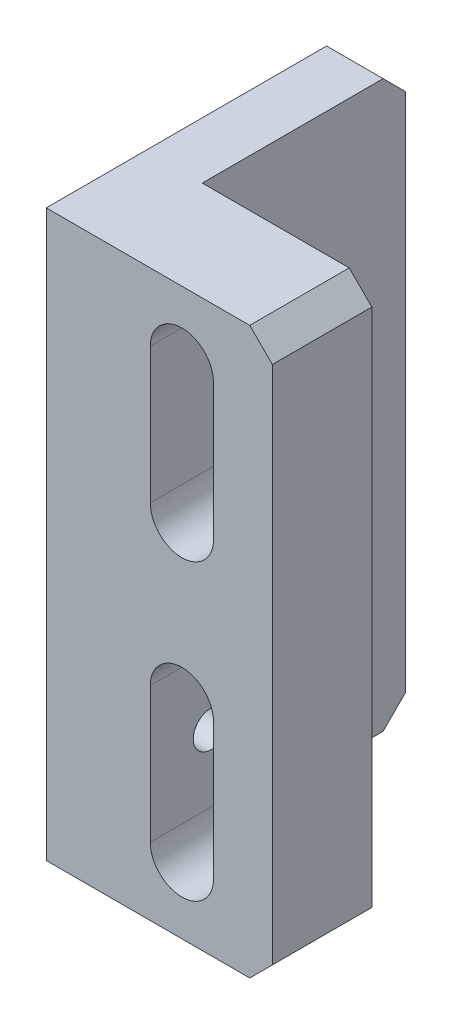
from build123d import *

# Parameters (mm, degrees)
SKETCH1_W             = 10
SKETCH1_H             = 13.4
BOSS_EXTRUDE1_DEPTH   = 25
CUT_EXTRUDE2_DEPTH    = 14
M2_TAPPED_HOLE1_D     = 1.6
M2_TAPPED_HOLE1_DEPTH = 5.2
M2_TAPPED_HOLE1_TIP   = 0.480688495
SKETCH7_W             = 9.563839575
SKETCH7_H             = 25
CUT_EXTRUDE3_DEPTH    = 9
CHAMFER1_SIZE         = 1


with BuildPart() as part:
    # Sketch1 → Boss-Extrude1 (new body)
    with BuildSketch(Plane(origin=(0, 0, 0), x_dir=(1, 0, 0), z_dir=(0, 1, 0))):
        with Locations((5, 6.7)):
            Rectangle(SKETCH1_W, SKETCH1_H)
    extrude(amount=BOSS_EXTRUDE1_DEPTH)

    # Q → Cut-Extrude2 (cut)
    with BuildSketch(Plane.XY):
        with BuildLine():
            Line((7.4, 22), (7.4, 16))
            ThreePointArc((7.4, 16), (6, 14.6), (4.6, 16))
            Line((4.6, 16), (4.6, 22))
            ThreePointArc((4.6, 22), (6, 23.4), (7.4, 22))
        make_face()
        with BuildLine():
            Line((7.4, 3), (7.4, 9))
            ThreePointArc((7.4, 9), (6, 10.4), (4.6, 9))
            Line((4.6, 9), (4.6, 3))
            ThreePointArc((4.6, 3), (6, 1.6), (7.4, 3))
        make_face()
    extrude(amount=-CUT_EXTRUDE2_DEPTH, mode=Mode.SUBTRACT)

    # M2 Tapped Hole1
    with Locations(Plane.ZY):
        with Locations((-10.7, 6), (-2.7, 6)):
            Hole(M2_TAPPED_HOLE1_D / 2, depth=M2_TAPPED_HOLE1_DEPTH)
            with Locations((0, 0, -(M2_TAPPED_HOLE1_DEPTH + M2_TAPPED_HOLE1_TIP / 2))):  # 118° drill point
                Cone(0, M2_TAPPED_HOLE1_D / 2, M2_TAPPED_HOLE1_TIP, mode=Mode.SUBTRACT)

    # Sketch7 → Cut-Extrude3 (cut)
    with BuildSketch(Plane(origin=(0, 0, -13.4), x_dir=(-1, 0, 0), z_dir=(0, 0, -1))):
        with Locations((-7.281919788, 12.5)):
            Rectangle(SKETCH7_W, SKETCH7_H)
    extrude(amount=-CUT_EXTRUDE3_DEPTH, mode=Mode.SUBTRACT)

    # Chamfer1
    chamfer1_edges = [part.edges().sort_by_distance(p)[0] for p in [
        (10, 25, -2.2),
        (10, 0, -2.2),
        (1.25, 0, -13.4),
        (1.25, 25, -13.4),
    ]]
    chamfer(chamfer1_edges, length=CHAMFER1_SIZE)


solid = part.part
